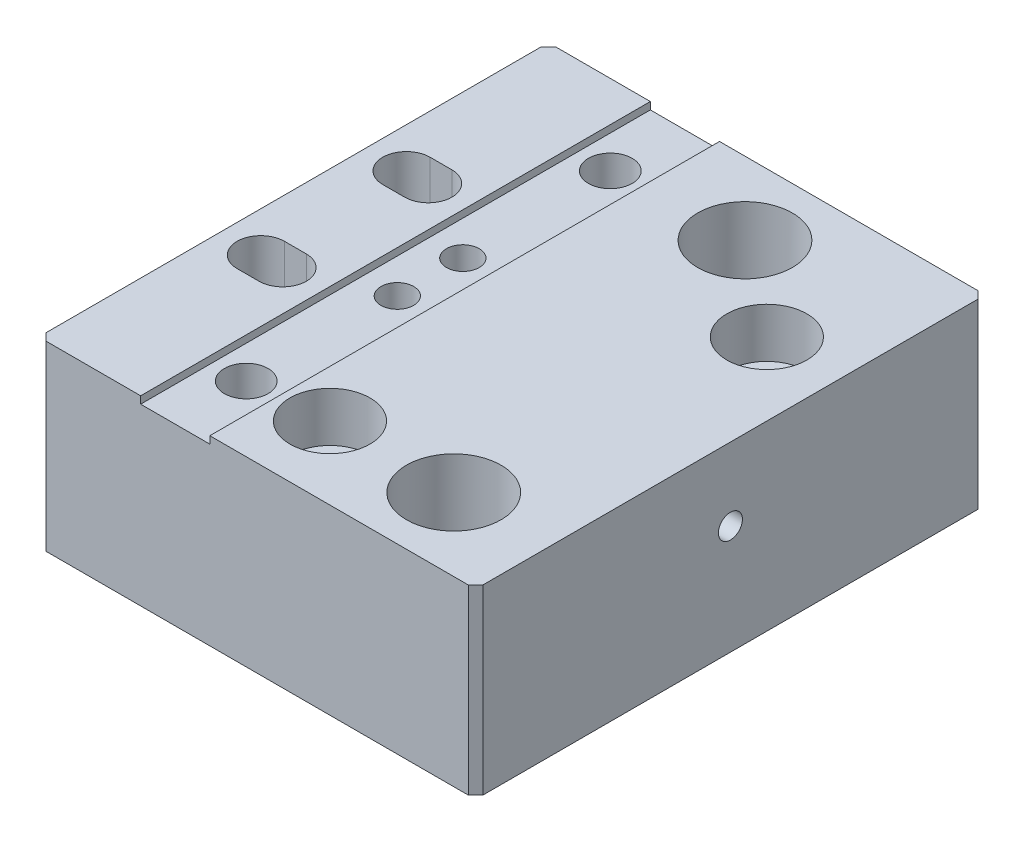
SolidWorks part; units mm, degrees
ref_plane "Front Plane" through (0, 0, 0) normal (0, 0, 1) x (1, 0, 0)
ref_plane "Top Plane" through (0, 0, 0) normal (0, 1, 0) x (1, 0, 0)
ref_plane "Right Plane" through (0, 0, 0) normal (1, 0, 0) x (0, 0, -1)
sketch "Sketch1" plane through (0, 0, 0) normal (0, 0, 1) x (1, 0, 0)
  line L1 (-30, 25) -> (30, 25)
  line L2 (-30, 25) -> (-30, 0)
  line L3 (-30, 0) -> (30, 0)
  line L4 (30, 25) -> (30, 0)
  dimension "D1" = 60
  dimension "D2" = 25
extrude "Boss-Extrude1" add sketch "Sketch1" along normal mid plane 70
sketch "Sketch2" plane through (0, 25, 0) normal (0, 1, 0) x (1, 0, 0)
  line L0 (-24.5, 10) -> (-21.5, 10) construction
  line L1 (-24.5, 13.25) -> (-21.5, 13.25)
  line L2 (-24.5, 6.75) -> (-21.5, 6.75)
  line L3 (-24.5, -10) -> (-21.5, -10) construction
  line L4 (-24.5, -6.75) -> (-21.5, -6.75)
  line L5 (-24.5, -13.25) -> (-21.5, -13.25)
  line L6 (-47.16, 0) -> (45.8019, 0) construction
  line L7 (-30, -35) -> (-30, 35) construction
  line L9 (30, -35) -> (-30, -35) construction
  arc A0 (-24.5, 13.25) -> (-24.5, 6.75) centre (-24.5, 10) ccw
  arc A1 (-21.5, 6.75) -> (-21.5, 13.25) centre (-21.5, 10) ccw
  arc A2 (-24.5, -6.75) -> (-24.5, -13.25) centre (-24.5, -10) ccw
  arc A3 (-21.5, -13.25) -> (-21.5, -6.75) centre (-21.5, -10) ccw
  circle A4 centre (7, 25) radius 6.5
  circle A5 centre (17, -25) radius 6.5
  point P2 (-23, 10)
  point P7 (-23, -10)
  dimension "D2" = 3.25
  dimension "D5" = 13
  dimension "D7" = 10
  dimension "D11" = 47
  dimension "D12" = 10
  dimension "D6" = 50
  dimension "D1" = 20
  dimension "D3" = 3
  dimension "D4" = 7
extrude "Cut-Extrude1" cut sketch "Sketch2" against normal through all
sketch "Sketch3" plane through (0, 0, 0) normal (0, -1, 0) x (1, 0, 0)
  circle A0 centre (17, 25) radius 9
  circle A1 centre (7, -25) radius 9
  dimension "D1" = 18
extrude "Cut-Extrude2" cut sketch "Sketch3" against normal blind 10
sketch "Sketch6" plane through (0, 25, 0) normal (0, 1, 0) x (-1, 0, 0)
  line L0 (-30, -35) -> (30, -35) construction
  line L1 (16, -35) -> (6.5, -35)
  line L2 (16, -35) -> (16, 35)
  line L3 (16, 35) -> (6.5, 35)
  line L4 (6.5, -35) -> (6.5, 35)
  line L6 (30, 35) -> (30, -35) construction
  line L7 (-30, 35) -> (30, 35) construction
  dimension "D1" = 14
  dimension "D2" = 9.5
extrude "Cut-Extrude3" cut sketch "Sketch6" against normal blind 1
hole_wizard "M4 Tapped Hole1" positions "Sketch8" profile "Sketch7" tap size "M4" standard "GB"
sketch "Sketch8" plane through (0, 24, 0) normal (0, 1, 0) x (-1, 0, 0)
  line L0 (52.3943, 0) -> (-47.4076, 0) construction
  line L2 (11.25, 35) -> (11.25, -35) construction
  line L3 (16, 35) -> (6.5, 35) construction
  line L4 (6.5, -35) -> (16, -35) construction
  point P0 (11.25, 4.5)
  point P1 (11.25, -4.5)
  dimension "D1" = 9
sketch "Sketch7" plane through (-11.25, 24, 4.5) normal (1, 0, 0) x (0, 0, 1)
  line L0 (0, 0) -> (0, 12.9914)
  line L1 (0, 12.9914) -> (1.65, 12)
  line L2 (1.65, 12) -> (1.65, 0)
  line L5 (1.65, 0) -> (0, 0)
  line L10 (0, 12.9914) -> (-1.65, 12) construction
  line L11 (0, -6.35) -> (0, 107.95) construction
  dimension "螺纹孔钻头直径" = 3.3
  dimension "螺纹孔钻头深度" = 12
  dimension "导头角度" = 118
cosmetic thread "Hole cosmetic thread1" parameters "D1"=8, "D2"=4
cosmetic thread "Hole cosmetic thread2" parameters "D1"=8, "D2"=4
sketch "Sketch10" plane through (0, 0, 0) normal (0, -1, 0) x (1, 0, 0)
  line L0 (-21.5, -10) -> (-30, -10) construction
  line L1 (-30, 35) -> (-30, -35) construction
  line L2 (-21.5, -16) -> (-30, -16)
  line L3 (-21.5, -4) -> (-30, -4)
  line L4 (-21.5, 10) -> (-30, 10) construction
  line L5 (-21.5, 4) -> (-30, 4)
  line L6 (-21.5, 16) -> (-30, 16)
  arc A0 (-21.5, -16) -> (-21.5, -4) centre (-21.5, -10) ccw
  arc A1 (-30, -4) -> (-30, -16) centre (-30, -10) ccw
  arc A2 (-21.5, 4) -> (-21.5, 16) centre (-21.5, 10) ccw
  arc A3 (-30, 16) -> (-30, 4) centre (-30, 10) ccw
  point P6 (-25.75, -10)
  point P12 (-25.75, 10)
  dimension "D1" = 12
extrude "Cut-Extrude4" cut sketch "Sketch10" against normal blind 7
hole_wizard "M5 Tapped Hole1" positions "Sketch14" profile "Sketch13" tap size "M5" standard "Gb"
sketch "Sketch14" plane through (0, 0, -35) normal (0, 0, -1) x (-1, 0, 0)
  line L0 (30, 0) -> (-30, 0) construction
  line L2 (-30, 0) -> (-30, 25) construction
  point P0 (-22.5, 19)
  point P2 (-22.5, 6)
  point P4 (22.5, 19)
  point P6 (22.5, 6)
  dimension "D1" = 13
  dimension "D2" = 6
  dimension "D3" = 45
  dimension "D4" = 7.5
sketch "Sketch13" plane through (22.5, 19, -35) normal (1, 0, 0) x (0, 1, 0)
  line L0 (0, 0) -> (0, 15.2618)
  line L1 (0, 15.2618) -> (2.1, 14)
  line L2 (2.1, 14) -> (2.1, 0)
  line L5 (2.1, 0) -> (0, 0)
  line L10 (0, 15.2618) -> (-2.1, 14) construction
  line L11 (0, -6.35) -> (0, 107.95) construction
  dimension "螺纹孔钻头直径" = 4.2
  dimension "螺纹孔钻头深度" = 14
  dimension "导头角度" = 118
cosmetic thread "Hole cosmetic thread4" parameters "D1"=10, "D2"=5
cosmetic thread "Hole cosmetic thread5" parameters "D1"=10, "D2"=5
cosmetic thread "Hole cosmetic thread6" parameters "D1"=10, "D2"=5
cosmetic thread "Hole cosmetic thread7" parameters "D1"=10, "D2"=5
hole_wizard "Hole size per socket head cap screw type2" positions "Sketch16" profile "Sketch15" counterbore size "M4" standard "Gb" end condition through all
sketch "Sketch16" plane through (0, 0, 0) normal (0, -1, 0) x (1, 0, 0)
  line L0 (-30, -16) -> (-30, -35) construction
  point P0 (-11.25, -4.5)
  point P2 (-11.25, 4.5)
  dimension "D1" = 9
  dimension "D2" = 4.5
  dimension "D3" = 18.75
sketch "Sketch15" plane through (-11.25, 0, -4.5) normal (1, 0, 0) x (0, 0, -1)
  line L0 (0, 0) -> (0, 25)
  line L1 (0, 25) -> (2.25, 25)
  line L3 (2.25, 25) -> (2.25, 4)
  line L4 (2.25, 4) -> (4, 4)
  line L5 (4, 4) -> (4, 0)
  line L7 (4, 0) -> (0, 0)
  line L11 (0, -6.35) -> (0, 107.95) construction
  dimension "通孔孔直径" = 4.5
  dimension "通孔孔深度" = 25
  dimension "柱形沉头孔直径" = 8
  dimension "柱形沉头孔深度" = 4
hole_wizard "M6 Tapped Hole1" positions "Sketch18" profile "Sketch17" tap size "M6" standard "Gb"
sketch "Sketch18" plane through (0, 0, 0) normal (0, -1, 0) x (1, 0, 0)
  line L0 (30, 35) -> (30, -35) construction
  line L1 (30, 35) -> (30, -35) construction
  point P0 (20, 0)
  point P2 (2, 0)
  point P11 (30, 0)
  dimension "D1" = 18
  dimension "D2" = 10
sketch "Sketch17" plane through (20, 0, 0) normal (1, 0, 0) x (0, 0, -1)
  line L0 (0, 0) -> (0, 16.5022)
  line L1 (0, 16.5022) -> (2.5, 15)
  line L2 (2.5, 15) -> (2.5, 0)
  line L5 (2.5, 0) -> (0, 0)
  line L10 (0, 16.5022) -> (-2.5, 15) construction
  line L11 (0, -6.35) -> (0, 107.95) construction
  dimension "螺纹孔钻头直径" = 5
  dimension "螺纹孔钻头深度" = 15
  dimension "导头角度" = 118
cosmetic thread "Hole cosmetic thread8" [suppressed] parameters "D1"=12, "D2"=6
cosmetic thread "Hole cosmetic thread9" [suppressed] parameters "D1"=12, "D2"=6
hole_wizard "Ø6.0 (6) Diameter Hole2" positions "Sketch20" profile "Sketch21" hole size "Ø6.0" standard "Gb" end condition up to next
sketch "Sketch20" plane through (0, 0, 0) normal (0, -1, 0) x (-1, 0, 0)
  line L0 (30, 0) -> (-34.2512, 0) construction
  line L1 (30, -35) -> (30, 35) construction
  point P0 (11.5, -25)
  point P2 (11.5, 25)
  dimension "D1" = 50
  dimension "D2" = 18.5
sketch "Sketch21" plane through (-11.5, 0, 25) normal (1, 0, 0) x (0, 0, -1)
  line L0 (0, 0) -> (0, 24)
  line L1 (0, 24) -> (3, 24)
  line L2 (3, 24) -> (3, 0)
  line L5 (3, 0) -> (0, 0)
  line L11 (0, -6.35) -> (0, 107.95) construction
  dimension "通孔孔直径" = 6
  dimension "通孔孔深度" = 24
hole_wizard "Hole size per socket head cap screw type3" positions "Sketch23" profile "Sketch22" counterbore size "M6" standard "Gb" end condition through all
sketch "Sketch23" plane through (0, 25, 0) normal (0, 1, 0) x (1, 0, 0)
  line L0 (30, -35) -> (-6.5, -35) construction
  line L1 (-30, -35) -> (-30, -16) construction
  point P0 (0, -25)
  point P2 (20, 15)
  dimension "D1" = 10
  dimension "D2" = 30
  dimension "D3" = 20
  dimension "D4" = 40
sketch "Sketch22" plane through (0, 25, 25) normal (1, 0, 0) x (0, 0, 1)
  line L0 (0, 0) -> (0, 25)
  line L1 (0, 25) -> (3.3, 25)
  line L3 (3.3, 25) -> (3.3, 6.8)
  line L4 (3.3, 6.8) -> (5.5, 6.8)
  line L5 (5.5, 6.8) -> (5.5, 0)
  line L7 (5.5, 0) -> (0, 0)
  line L11 (0, -6.35) -> (0, 107.95) construction
  dimension "通孔孔直径" = 6.6
  dimension "通孔孔深度" = 25
  dimension "柱形沉头孔直径" = 11
  dimension "柱形沉头孔深度" = 6.8
hole_wizard "M4 Tapped Hole2" positions "Sketch25" profile "Sketch24" tap size "M4" standard "Gb"
sketch "Sketch25" plane through (30, 0, 0) normal (1, 0, 0) x (0, 0, -1)
  line L0 (-35, 25) -> (35, 25) construction
  point P0 (0, 15)
  dimension "D1" = 10
sketch "Sketch24" plane through (30, 15, 0) normal (0, 1, 0) x (0, 0, -1)
  line L0 (0, 0) -> (0, 15.9914)
  line L1 (0, 15.9914) -> (1.65, 15)
  line L2 (1.65, 15) -> (1.65, 0)
  line L5 (1.65, 0) -> (0, 0)
  line L10 (0, 15.9914) -> (-1.65, 15) construction
  line L11 (0, -6.35) -> (0, 107.95) construction
  dimension "螺纹孔钻头直径" = 3.3
  dimension "螺纹孔钻头深度" = 15
  dimension "导头角度" = 118
cosmetic thread "Hole cosmetic thread10" parameters "D1"=8, "D2"=4
chamfer "Chamfer1" distance 1 angle 45 5 edges at (30, 12.5, -35) (-30, 12.5, -35) (-30, 12.5, 35) (30, 12.5, 35) (-30, 25, 0)
